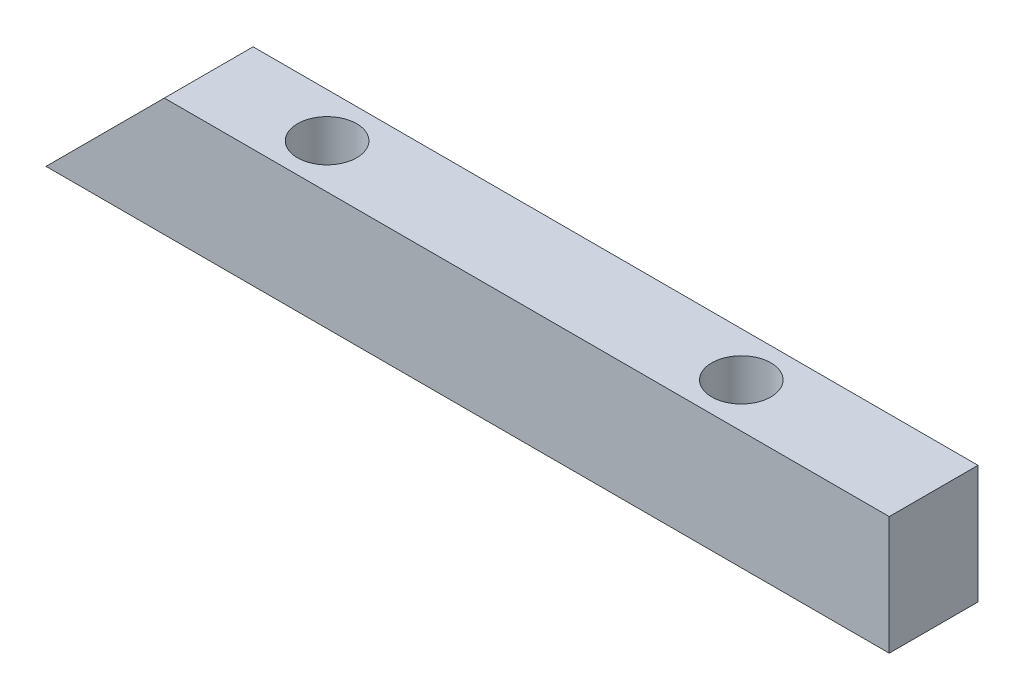
from build123d import *

# Parameters (mm, degrees)
SKETCH_1_W          = 270
SKETCH_1_H          = 30
EXTRUDE_1_DEPTH     = 40
SKETCH_2_R          = 10
CUT_EXTRUDE_2_DEPTH = 30
SKETCH_3_W          = 30
SKETCH_3_H          = 40
EXTRUDE_2_DEPTH     = 15
CUT_EXTRUDE_3_DEPTH = 159.113883008


with BuildPart() as part:
    # 草图1 → 凸台-拉伸1 (new body)
    with BuildSketch(Plane(origin=(0, 0, 0), x_dir=(1, 0, 0), z_dir=(0, 1, 0))):
        Rectangle(SKETCH_1_W, SKETCH_1_H)
    extrude(amount=EXTRUDE_1_DEPTH)

    # 草图2 → 切除-拉伸2 (cut)
    with BuildSketch(Plane(origin=(0, 40, 0), x_dir=(1, 0, 0), z_dir=(0, 1, 0))):
        with Locations(Location((70, 0, 0), (0, 0, 270))):
            Circle(SKETCH_2_R)
        with Locations(Location((-70, 0, 0), (0, 0, 90))):
            Circle(SKETCH_2_R)
    extrude(amount=-CUT_EXTRUDE_2_DEPTH, mode=Mode.SUBTRACT)

    # 草图3 → 凸台-拉伸2 (add)
    with BuildSketch(Plane.ZY.offset(135)):
        with Locations((0, 20)):
            Rectangle(SKETCH_3_W, SKETCH_3_H)
    extrude(amount=EXTRUDE_2_DEPTH)

    # 草图4 → 切除-拉伸3 (cut, through all)
    with BuildSketch(Plane.XY.offset(15)):
        Polygon((-150, 0), (-110, 40), (-150, 40), align=None)
    extrude(amount=-CUT_EXTRUDE_3_DEPTH, mode=Mode.SUBTRACT)


solid = part.part
